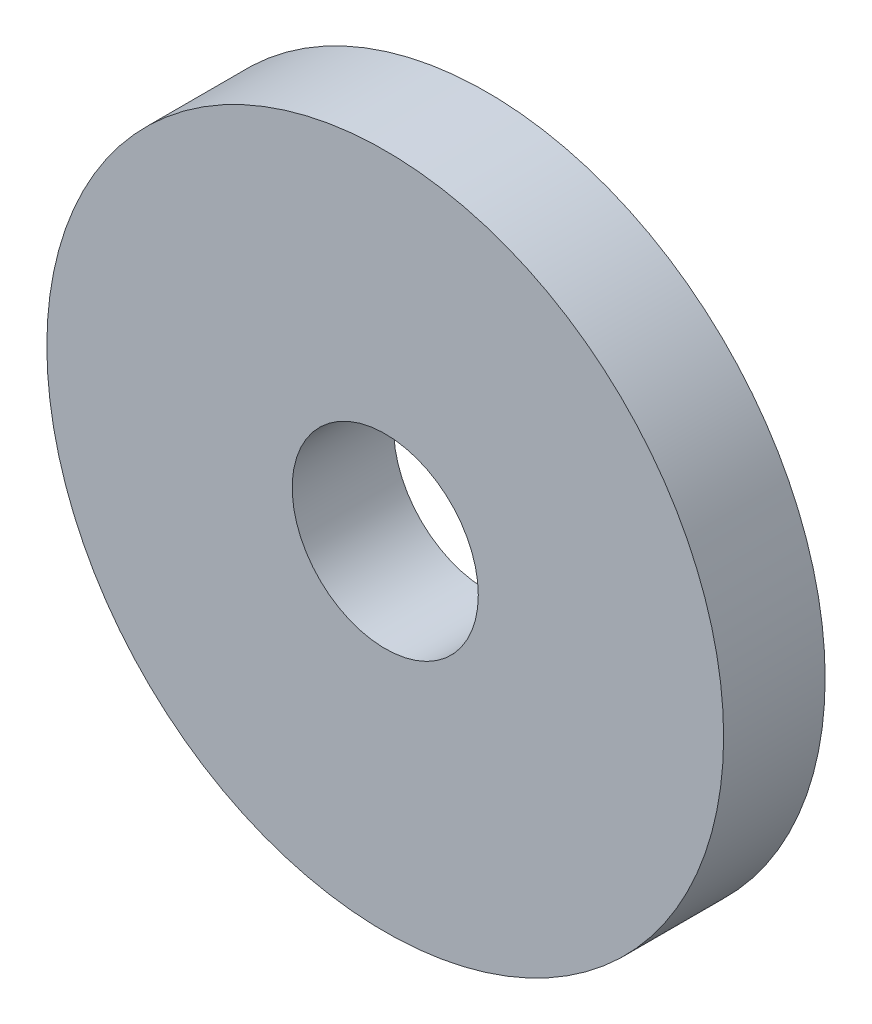
SolidWorks part; units mm, degrees
material "Q235B"
ref_plane "Front Plane" through (0, 0, 0) normal (0, 0, 1) x (1, 0, 0)
ref_plane "Top Plane" through (0, 0, 0) normal (0, 1, 0) x (1, 0, 0)
ref_plane "Right Plane" through (0, 0, 0) normal (1, 0, 0) x (0, 0, -1)
sketch "Sketch1" plane through (0, 0, 0) normal (0, 0, 1) x (1, 0, 0)
  circle A0 centre (0, 0) radius 40
  circle A1 centre (0, 0) radius 11
  dimension "D1" = 80
  dimension "D2" = 22
extrude "Boss-Extrude1" add sketch "Sketch1" along normal blind 12
